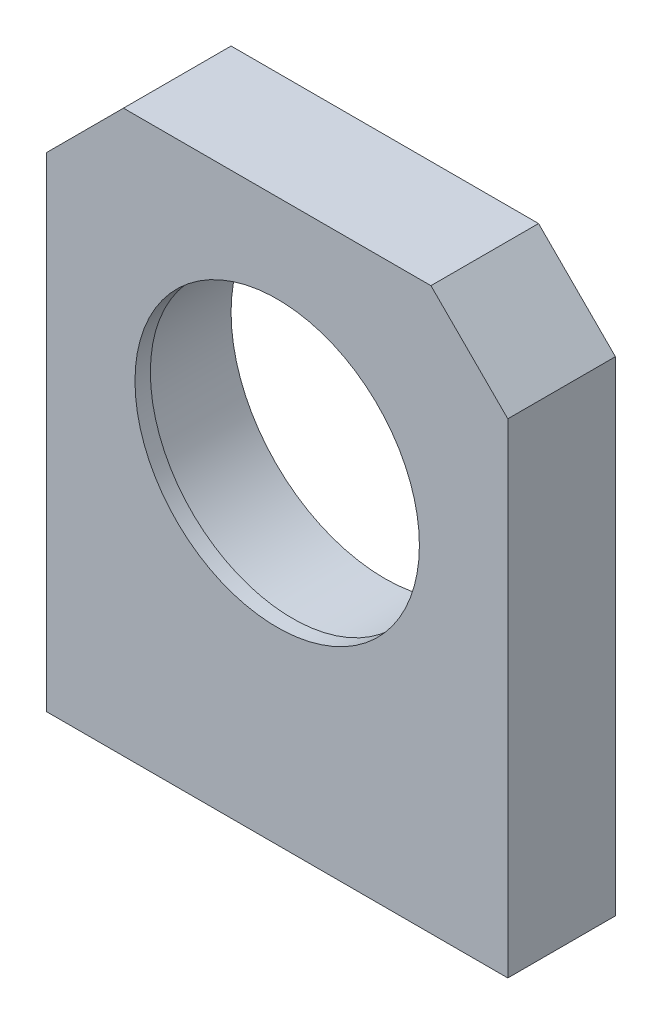
from build123d import *

# Parameters (mm, degrees)
SKETCH_1_W             = 60
SKETCH_1_H             = 73
SKETCH_1_R             = 20
EXTRUDE_1_DEPTH        = 7
EXTRUDE_START          = -2
SKETCH_2_R             = 20
SKETCH_2_R_2           = 18.5
EXTRUDE_2_DEPTH        = 2
CHAMFER_1_SIZE         = 10
HOLE_WIZARD_M6_1_D     = 5
HOLE_WIZARD_M6_1_DEPTH = 14
HOLE_WIZARD_M6_1_TIP   = 1.502151548


with BuildPart() as part:
    # 草图1 → 凸台-拉伸1 (new, symmetric)
    with BuildSketch(Plane.XY):
        Rectangle(SKETCH_1_W, SKETCH_1_H)
        with Locations((0, 6.5)):
            Circle(SKETCH_1_R, mode=Mode.SUBTRACT)
    extrude(amount=EXTRUDE_1_DEPTH, both=True)

    # 草图2 → 凸台-拉伸2 (add)
    with BuildSketch(Plane.XY.offset(7).offset(EXTRUDE_START)):
        with Locations((0, 6.5)):
            Circle(SKETCH_2_R)
        with Locations((0, 6.5)):
            Circle(SKETCH_2_R_2, mode=Mode.SUBTRACT)
    extrude(amount=EXTRUDE_2_DEPTH)

    # 倒角1
    chamfer_1_edges = [part.edges().sort_by_distance(p)[0] for p in [
        (-30, 36.5, 0),
        (30, 36.5, 0),
    ]]
    chamfer(chamfer_1_edges, length=CHAMFER_1_SIZE)

    # M6 螺纹孔1
    with Locations(Plane(origin=(-24, -36.5, 0), x_dir=(0, 0, -1), z_dir=(0, -1, 0))):
        with Locations((0, 0), (0, 48)):
            Hole(HOLE_WIZARD_M6_1_D / 2, depth=HOLE_WIZARD_M6_1_DEPTH)
            with Locations((0, 0, -(HOLE_WIZARD_M6_1_DEPTH + HOLE_WIZARD_M6_1_TIP / 2))):  # 118° drill point
                Cone(0, HOLE_WIZARD_M6_1_D / 2, HOLE_WIZARD_M6_1_TIP, mode=Mode.SUBTRACT)


solid = part.part
